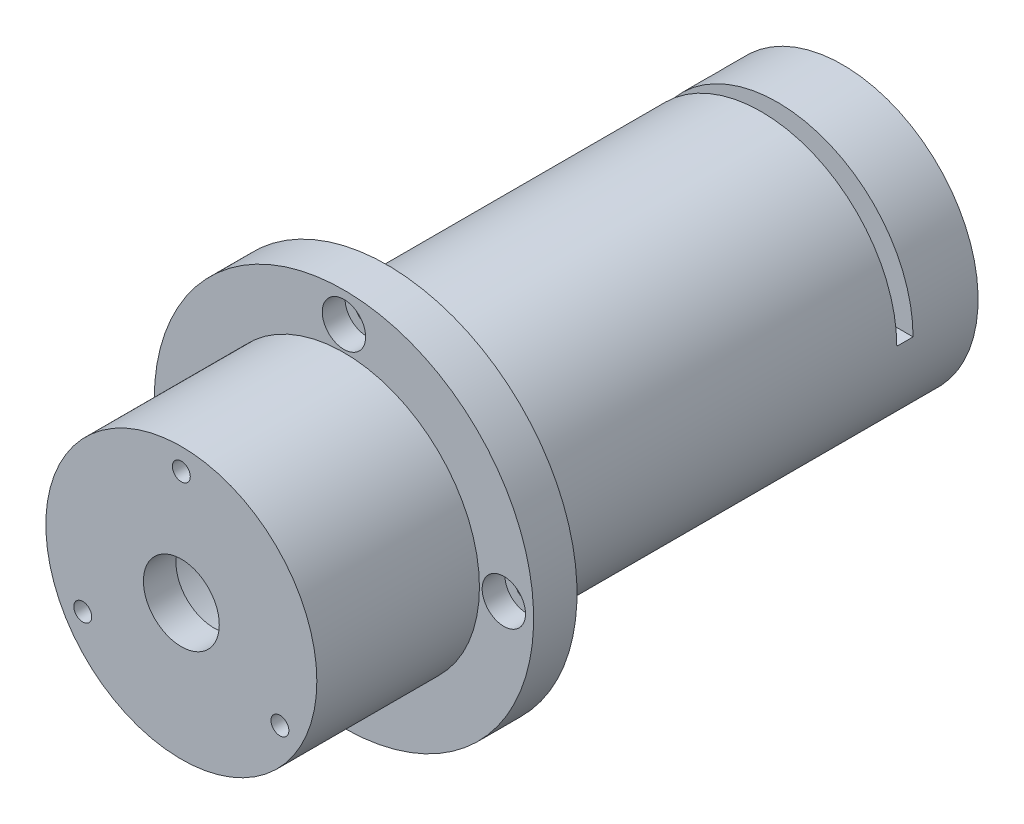
from build123d import *

# Parameters (mm, degrees)
SKETCH_2_R             = 35
EXTRUDE_1_DEPTH        = 122
SKETCH_3_R             = 7
CUT_EXTRUDE_1_DEPTH    = 132.658649545
SKETCH_4_R             = 17.5
CUT_EXTRUDE_2_DEPTH    = 116
SKETCH_5_OUTSIDE_W     = 103.422
SKETCH_5_OUTSIDE_H     = 103.422
SKETCH_5_OUTSIDE_R     = 25
CUT_EXTRUDE_3_DEPTH    = 30
SKETCH_6_OUTSIDE_W     = 103.422
SKETCH_6_OUTSIDE_H     = 103.422
SKETCH_6_OUTSIDE_R     = 25
CUT_EXTRUDE_4_DEPTH    = 84
SKETCH_7_R             = 2.1
CUT_EXTRUDE_5_DEPTH    = 105.470091414
SKETCH_8_R             = 4
CUT_EXTRUDE_6_DEPTH    = 4.2
HOLE_WIZARD_M4_1_D     = 3.3
HOLE_WIZARD_M4_1_DEPTH = 10.5
HOLE_WIZARD_M4_1_TIP   = 0.991420021
SKETCH_19_W            = 12.931297241
SKETCH_19_H            = 3
CUT_EXTRUDE_7_DEPTH    = 15
SKETCH_20_W            = 3
SKETCH_20_H            = 28.427665472
CUT_EXTRUDE_8_DEPTH    = 141.388745988
SKETCH_21_R            = 4
CUT_EXTRUDE_9_DEPTH    = 18
SKETCH_22_R            = 2.25
CUT_EXTRUDE_10_DEPTH   = 22
HOLE_WIZARD_M4_3_D     = 3.3


with BuildPart() as part:
    # 草图2 → 凸台-拉伸1 (new body)
    with BuildSketch(Plane.XY):
        with Locations(Location((0, 0, 0), (0, 0, 180))):
            Circle(SKETCH_2_R)
    extrude(amount=EXTRUDE_1_DEPTH)

    # 草图3 → 切除-拉伸1 (cut, through all)
    with BuildSketch(Plane.XY.offset(122)):
        Circle(SKETCH_3_R)
    extrude(amount=-CUT_EXTRUDE_1_DEPTH, mode=Mode.SUBTRACT)

    # 草图4 → 切除-拉伸2 (cut)
    with BuildSketch(Plane(origin=(0, 0, 0), x_dir=(-1, 0, 0), z_dir=(0, 0, -1))):
        Circle(SKETCH_4_R)
    extrude(amount=-CUT_EXTRUDE_2_DEPTH, mode=Mode.SUBTRACT)

    # 草图5 outside → 切除-拉伸3 (cut)
    with BuildSketch(Plane.XY.offset(122)):
        Rectangle(SKETCH_5_OUTSIDE_W, SKETCH_5_OUTSIDE_H)
        Circle(SKETCH_5_OUTSIDE_R, mode=Mode.SUBTRACT)
    extrude(amount=-CUT_EXTRUDE_3_DEPTH, mode=Mode.SUBTRACT)

    # 草图6 outside → 切除-拉伸4 (cut)
    with BuildSketch(Plane(origin=(0, 0, 0), x_dir=(-1, 0, 0), z_dir=(0, 0, -1))):
        Rectangle(SKETCH_6_OUTSIDE_W, SKETCH_6_OUTSIDE_H)
        with Locations(Location((0, 0, 0), (0, 0, 180))):
            Circle(SKETCH_6_OUTSIDE_R, mode=Mode.SUBTRACT)
    extrude(amount=-CUT_EXTRUDE_4_DEPTH, mode=Mode.SUBTRACT)

    # 草图7 → 切除-拉伸5 (cut, through all)
    with BuildSketch(Plane.XY.offset(92)):
        with Locations((0, 29.5)):
            Circle(SKETCH_7_R)
        with Locations((29.5, 0)):
            Circle(SKETCH_7_R)
        with Locations((0, -29.5)):
            Circle(SKETCH_7_R)
        with Locations((-29.5, 0)):
            Circle(SKETCH_7_R)
    extrude(amount=-CUT_EXTRUDE_5_DEPTH, mode=Mode.SUBTRACT)

    # 草图8 → 切除-拉伸6 (cut)
    with BuildSketch(Plane.XY.offset(92)):
        with Locations((0, 29.5)):
            Circle(SKETCH_8_R)
        with Locations((-29.5, 0)):
            Circle(SKETCH_8_R)
        with Locations((29.5, 0)):
            Circle(SKETCH_8_R)
        with Locations((0, -29.5)):
            Circle(SKETCH_8_R)
    extrude(amount=-CUT_EXTRUDE_6_DEPTH, mode=Mode.SUBTRACT)

    # M4 螺纹孔1
    with Locations(Plane(origin=(18.186533479, -10.5, 122), x_dir=(1, 0, 0), z_dir=(0, 0, 1))):
        with Locations((0, 0), (-36.373066958, 0), (-18.186533479, 31.5)):
            Hole(HOLE_WIZARD_M4_1_D / 2, depth=HOLE_WIZARD_M4_1_DEPTH)
            with Locations((0, 0, -(HOLE_WIZARD_M4_1_DEPTH + HOLE_WIZARD_M4_1_TIP / 2))):  # 118° drill point
                Cone(0, HOLE_WIZARD_M4_1_D / 2, HOLE_WIZARD_M4_1_TIP, mode=Mode.SUBTRACT)

    # 草图19 → 切除-拉伸7 (cut)
    with BuildSketch(Plane(origin=(0, 0, 0), x_dir=(-1, 0, 0), z_dir=(0, 0, -1))):
        with Locations((20.220472236, 1.5)):
            Rectangle(SKETCH_19_W, SKETCH_19_H)
    extrude(amount=-CUT_EXTRUDE_7_DEPTH, mode=Mode.SUBTRACT)

    # 草图20 → 切除-拉伸8 (cut, through all)
    with BuildSketch(Plane(origin=(-25, 0, 0), x_dir=(0, 0, -1), z_dir=(1, 0, 0))):
        with Locations((-13.5, 14.213832736)):
            Rectangle(SKETCH_20_W, SKETCH_20_H)
    extrude(amount=CUT_EXTRUDE_8_DEPTH, mode=Mode.SUBTRACT)

    # 草图21 → 切除-拉伸9 (cut)
    with BuildSketch(Plane(origin=(0, 25, 0), x_dir=(-1, 0, 0), z_dir=(0, 1, 0))):
        with Locations((21, 6)):
            Circle(SKETCH_21_R)
    extrude(amount=-CUT_EXTRUDE_9_DEPTH, mode=Mode.SUBTRACT)

    # 草图22 → 切除-拉伸10 (cut)
    with BuildSketch(Plane(origin=(0, 25, 0), x_dir=(-1, 0, 0), z_dir=(0, 1, 0))):
        with Locations(Location((21, 6, 0), (0, 0, 90))):
            Circle(SKETCH_22_R)
    extrude(amount=-CUT_EXTRUDE_10_DEPTH, mode=Mode.SUBTRACT)

    # M4 螺纹孔3 (through all)
    with Locations(Plane(origin=(-21, 0, 6), x_dir=(0, 0, 1), z_dir=(0, 1, 0))):
        with Locations((0, 0)):
            Hole(HOLE_WIZARD_M4_3_D / 2)


solid = part.part
